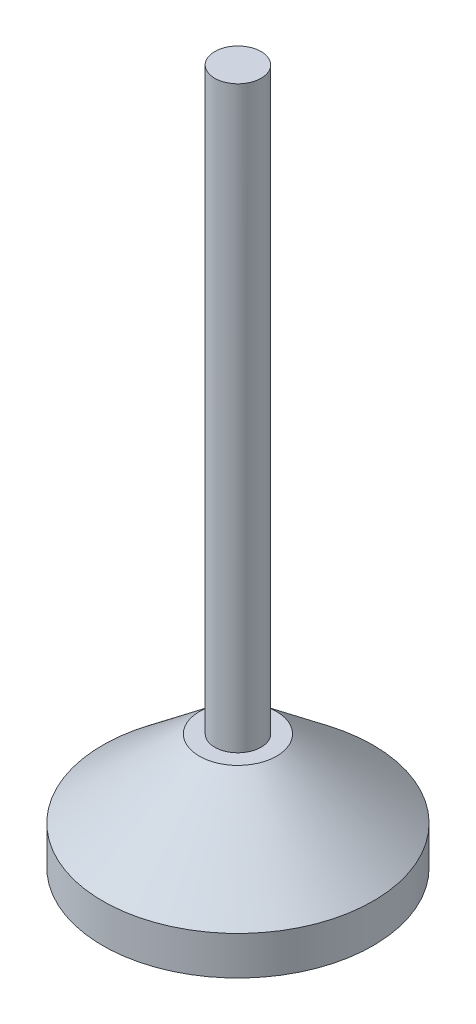
SolidWorks part; units mm, degrees
ref_plane "前视基准面" through (0, 0, 0) normal (0, 0, 1) x (1, 0, 0)
ref_plane "上视基准面" through (0, 0, 0) normal (0, 1, 0) x (1, 0, 0)
ref_plane "右视基准面" through (0, 0, 0) normal (1, 0, 0) x (0, 0, -1)
sketch "草图1" plane through (0, 0, 0) normal (0, 1, 0) x (1, 0, 0)
  circle A0 centre (0, 0) radius 6
  dimension "D1" = 12
extrude "凸台-拉伸1" add sketch "草图1" along normal blind 150
sketch "草图2" plane through (0, 0, 0) normal (0, -1, 0) x (1, 0, 0)
  circle A0 centre (0, 0) radius 35
  dimension "D1" = 70
extrude "凸台-拉伸2" add sketch "草图2" along normal blind 30
chamfer "倒角1" distance 25 distance2 20 1 edges at (0, 0, -35)
